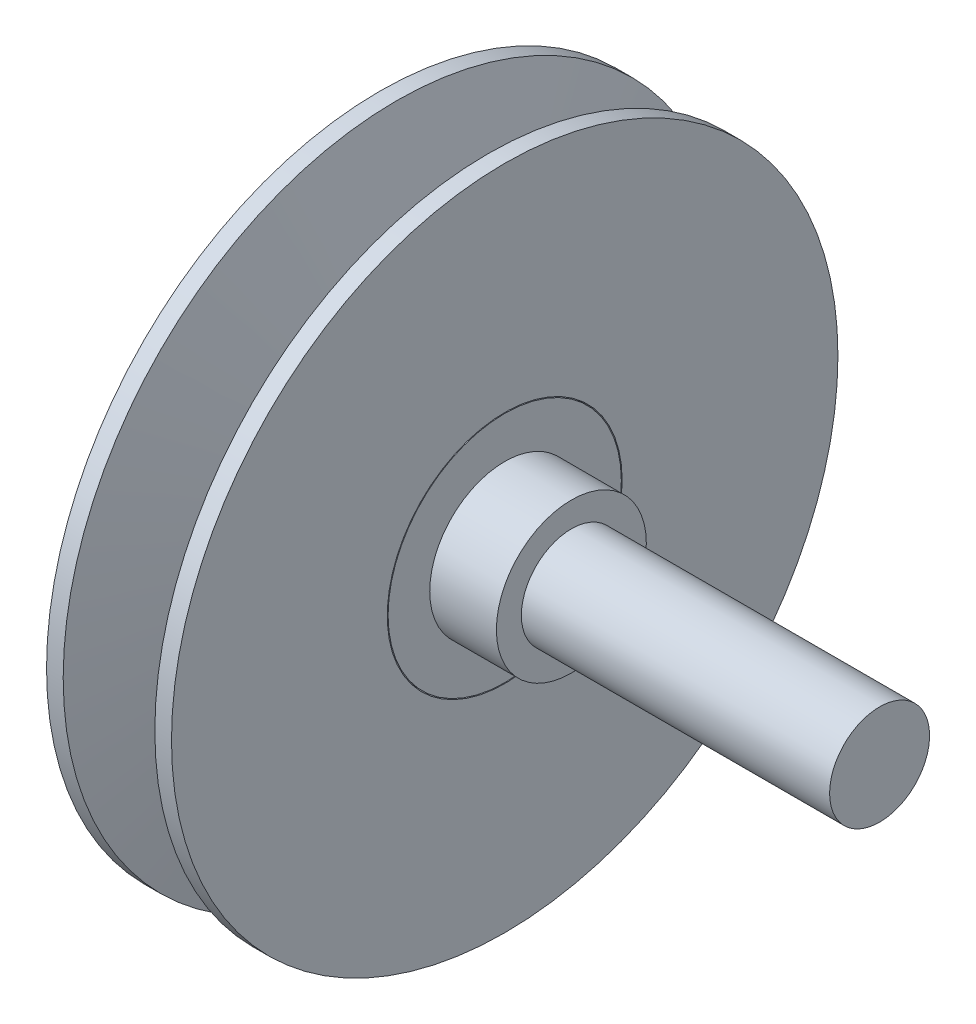
from build123d import *

# Parameters (mm, degrees)
SKETCH2_R           = 6
CUT_EXTRUDE1_DEPTH  = 59.523499554
SKETCH3_R           = 14.1
SKETCH3_R_2         = 14
CUT_EXTRUDE2_DEPTH  = 3
CUT_EXTRUDE3_START  = -3
SKETCH4_R           = 14.1
SKETCH4_R_2         = 14
CUT_EXTRUDE3_DEPTH  = 3
SKETCH5_R           = 6
BOSS_EXTRUDE1_DEPTH = 45
SKETCH6_R           = 9
BOSS_EXTRUDE2_DEPTH = 8


with BuildPart() as part:
    # Sketch1 → Revolve1 (revolve)
    with BuildSketch(Plane.XY, mode=Mode.PRIVATE) as revolve1_sk:
        with BuildLine():
            Line((0, 0), (0, 40))
            Line((0, 40), (2, 40))
            Line((2, 40), (5.047051836, 24.51725234))
            ThreePointArc((5.047051836, 24.51725234), (7.5, 22.5), (9.952948164, 24.51725234))
            Line((9.952948164, 24.51725234), (13, 40))
            Line((13, 40), (15, 40))
            Line((15, 40), (15, 0))
            Line((15, 0), (0, 0))
        make_face()
    revolve(revolve1_sk.sketch.rotate(Axis((0, 0, 0), (1, 0, 0)), 90), axis=Axis((0, 0, 0), (1, 0, 0)))

    # Sketch2 → Cut-Extrude1 (cut, through all)
    with BuildSketch(Plane.ZY):
        Circle(SKETCH2_R)
    extrude(amount=-CUT_EXTRUDE1_DEPTH, mode=Mode.SUBTRACT)

    # Sketch3 → Cut-Extrude2 (cut)
    with BuildSketch(Plane.ZY):
        Circle(SKETCH3_R)
        Circle(SKETCH3_R_2, mode=Mode.SUBTRACT)
    extrude(amount=-CUT_EXTRUDE2_DEPTH, mode=Mode.SUBTRACT)

    # Sketch4 → Cut-Extrude3 (cut)
    with BuildSketch(Plane(origin=(15, 0, 0), x_dir=(0, 0, -1), z_dir=(1, 0, 0)).offset(CUT_EXTRUDE3_START)):
        with Locations(Location((0, 0, 0), (0, 0, 180))):
            Circle(SKETCH4_R)
        with Locations(Location((0, 0, 0), (0, 0, 180))):
            Circle(SKETCH4_R_2, mode=Mode.SUBTRACT)
    extrude(amount=CUT_EXTRUDE3_DEPTH, mode=Mode.SUBTRACT)



with BuildPart() as body_2:
    # Sketch5 → Boss-Extrude1 (new body)
    with BuildSketch(Plane(origin=(15, 0, 0), x_dir=(0, 0, -1), z_dir=(1, 0, 0))):
        with Locations(Location((0, 0, 0), (0, 0, 180))):
            Circle(SKETCH5_R)
    extrude(amount=BOSS_EXTRUDE1_DEPTH)


with BuildPart() as part_1:
    add(part.part)

    add(body_2.part)  # Boss-Extrude2 merges body 2
    # Sketch6 → Boss-Extrude2 (add)
    with BuildSketch(Plane(origin=(15, 0, 0), x_dir=(0, 0, -1), z_dir=(1, 0, 0))):
        with Locations(Location((0, 0, 0), (0, 0, 180))):
            Circle(SKETCH6_R)
    extrude(amount=BOSS_EXTRUDE2_DEPTH)


solid = part_1.part
